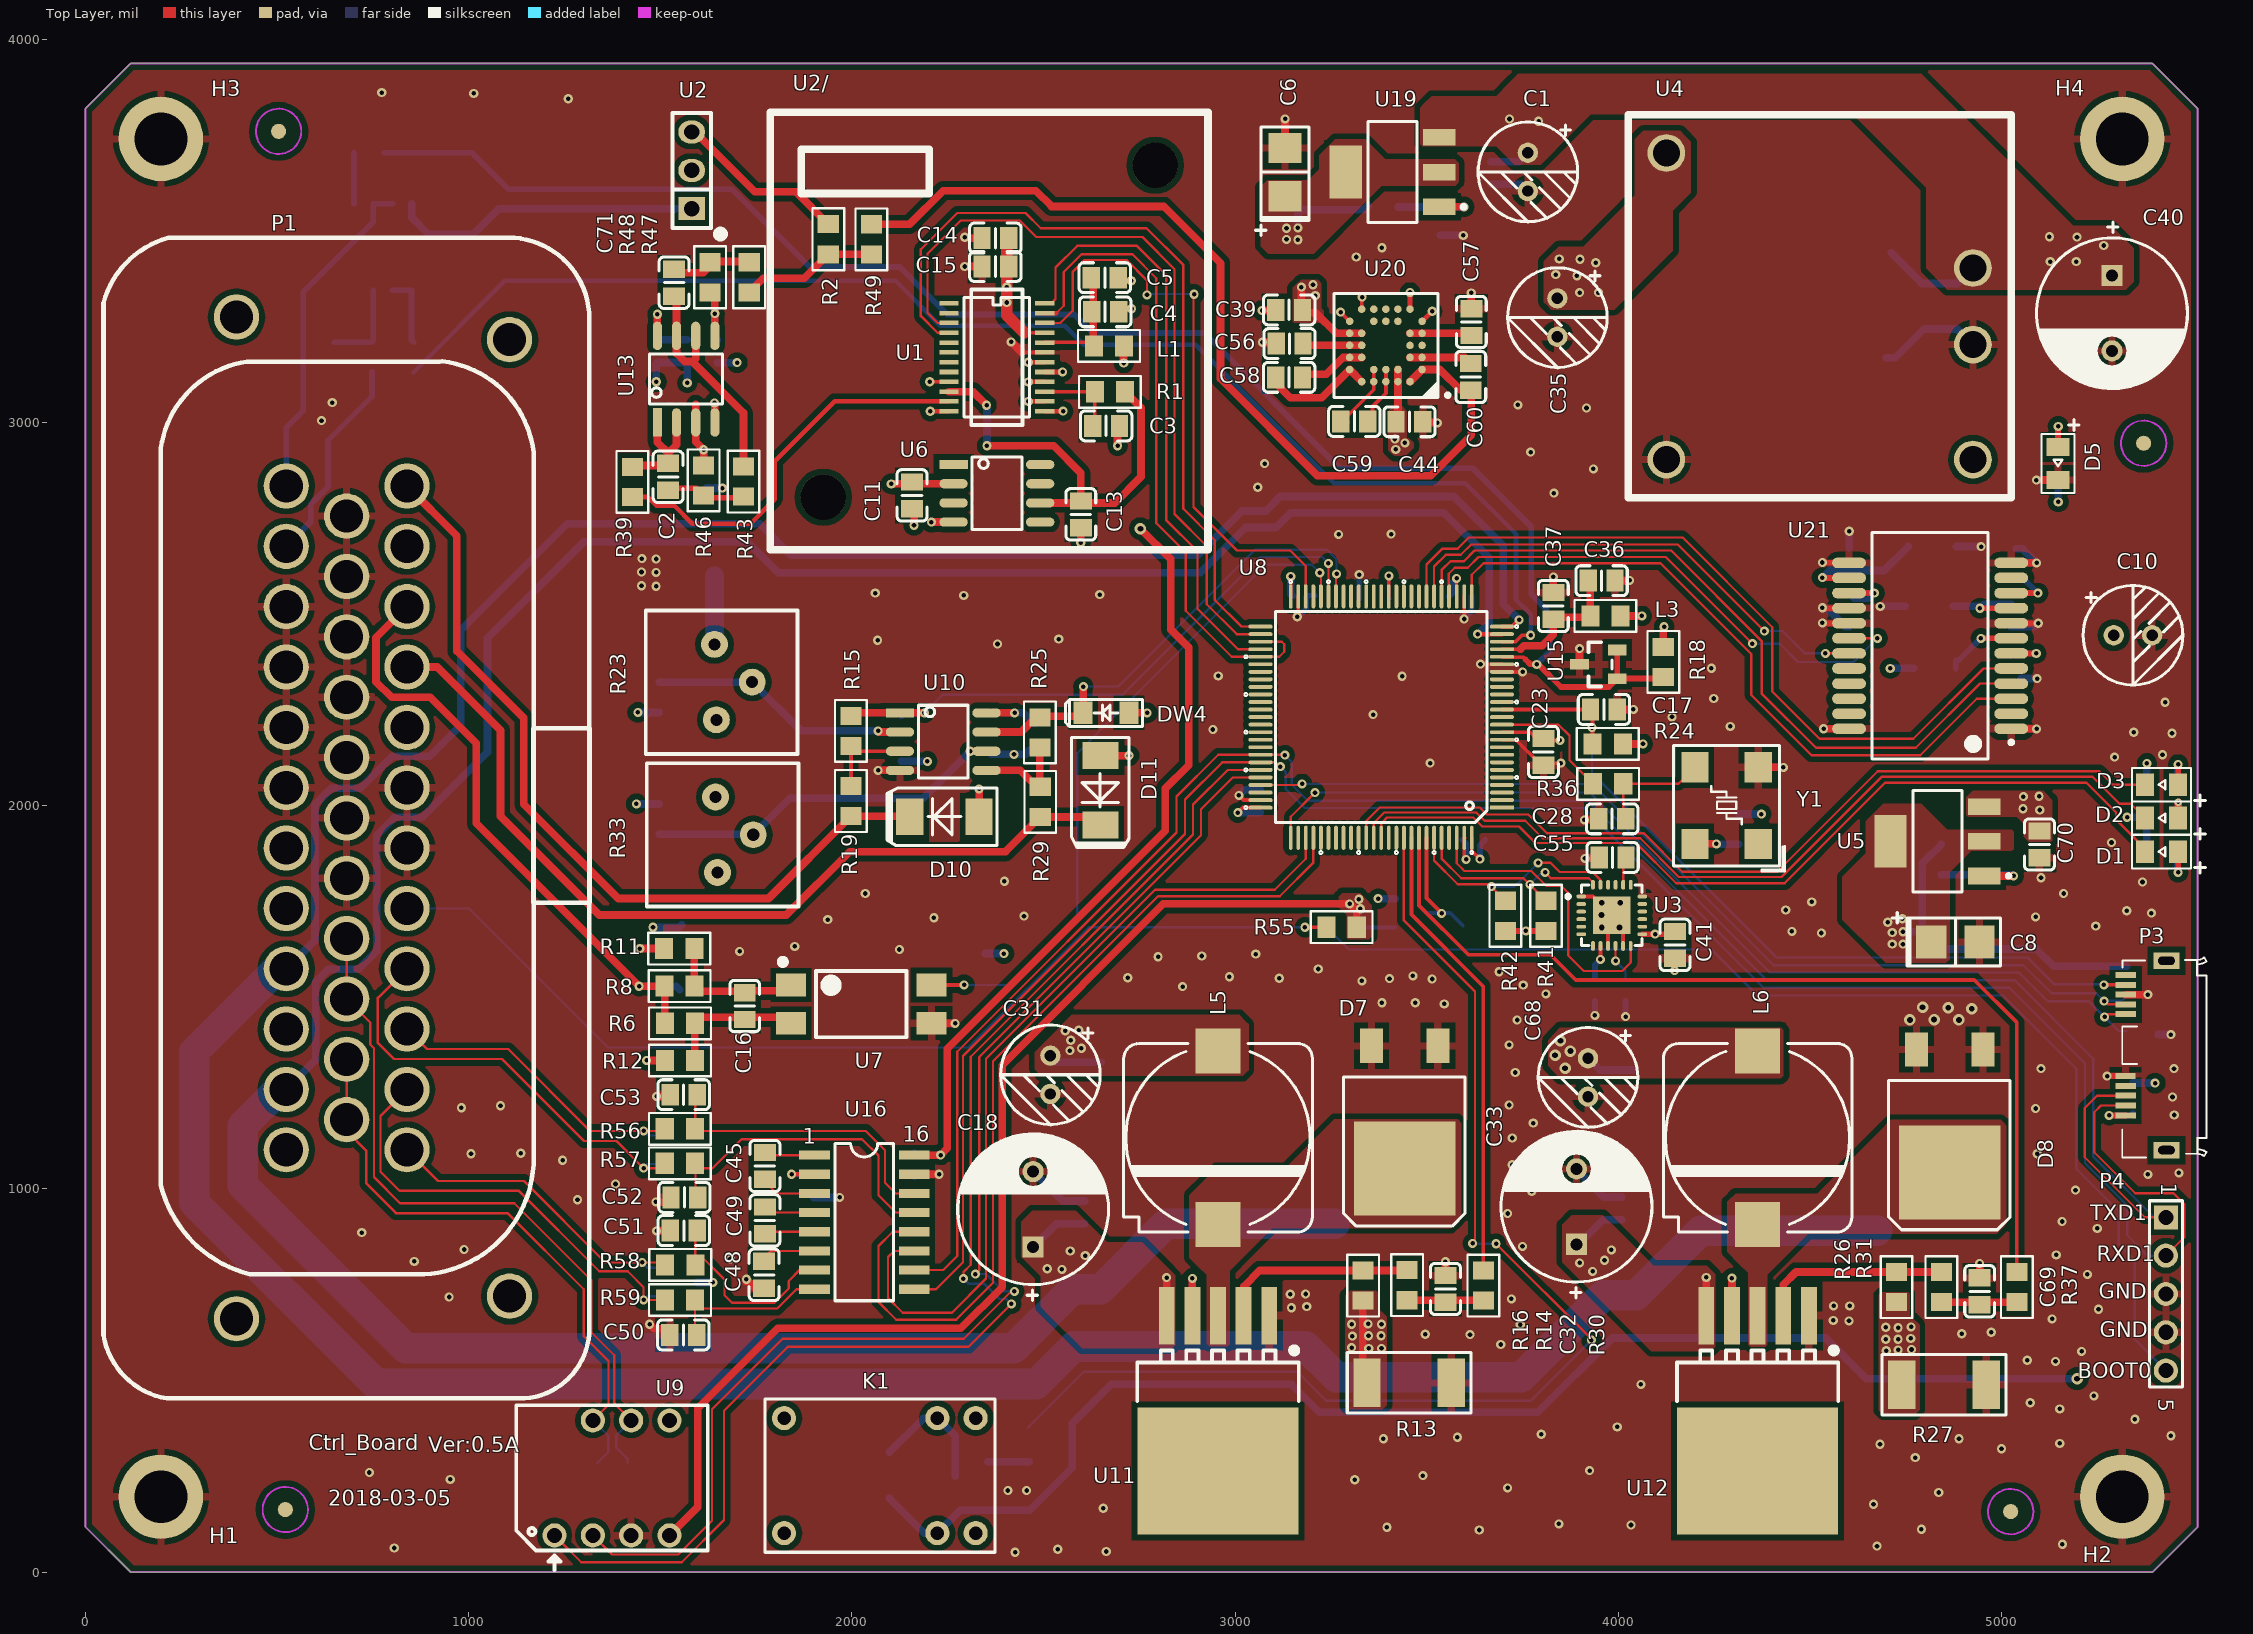
[diagram p0: Top Layer view]
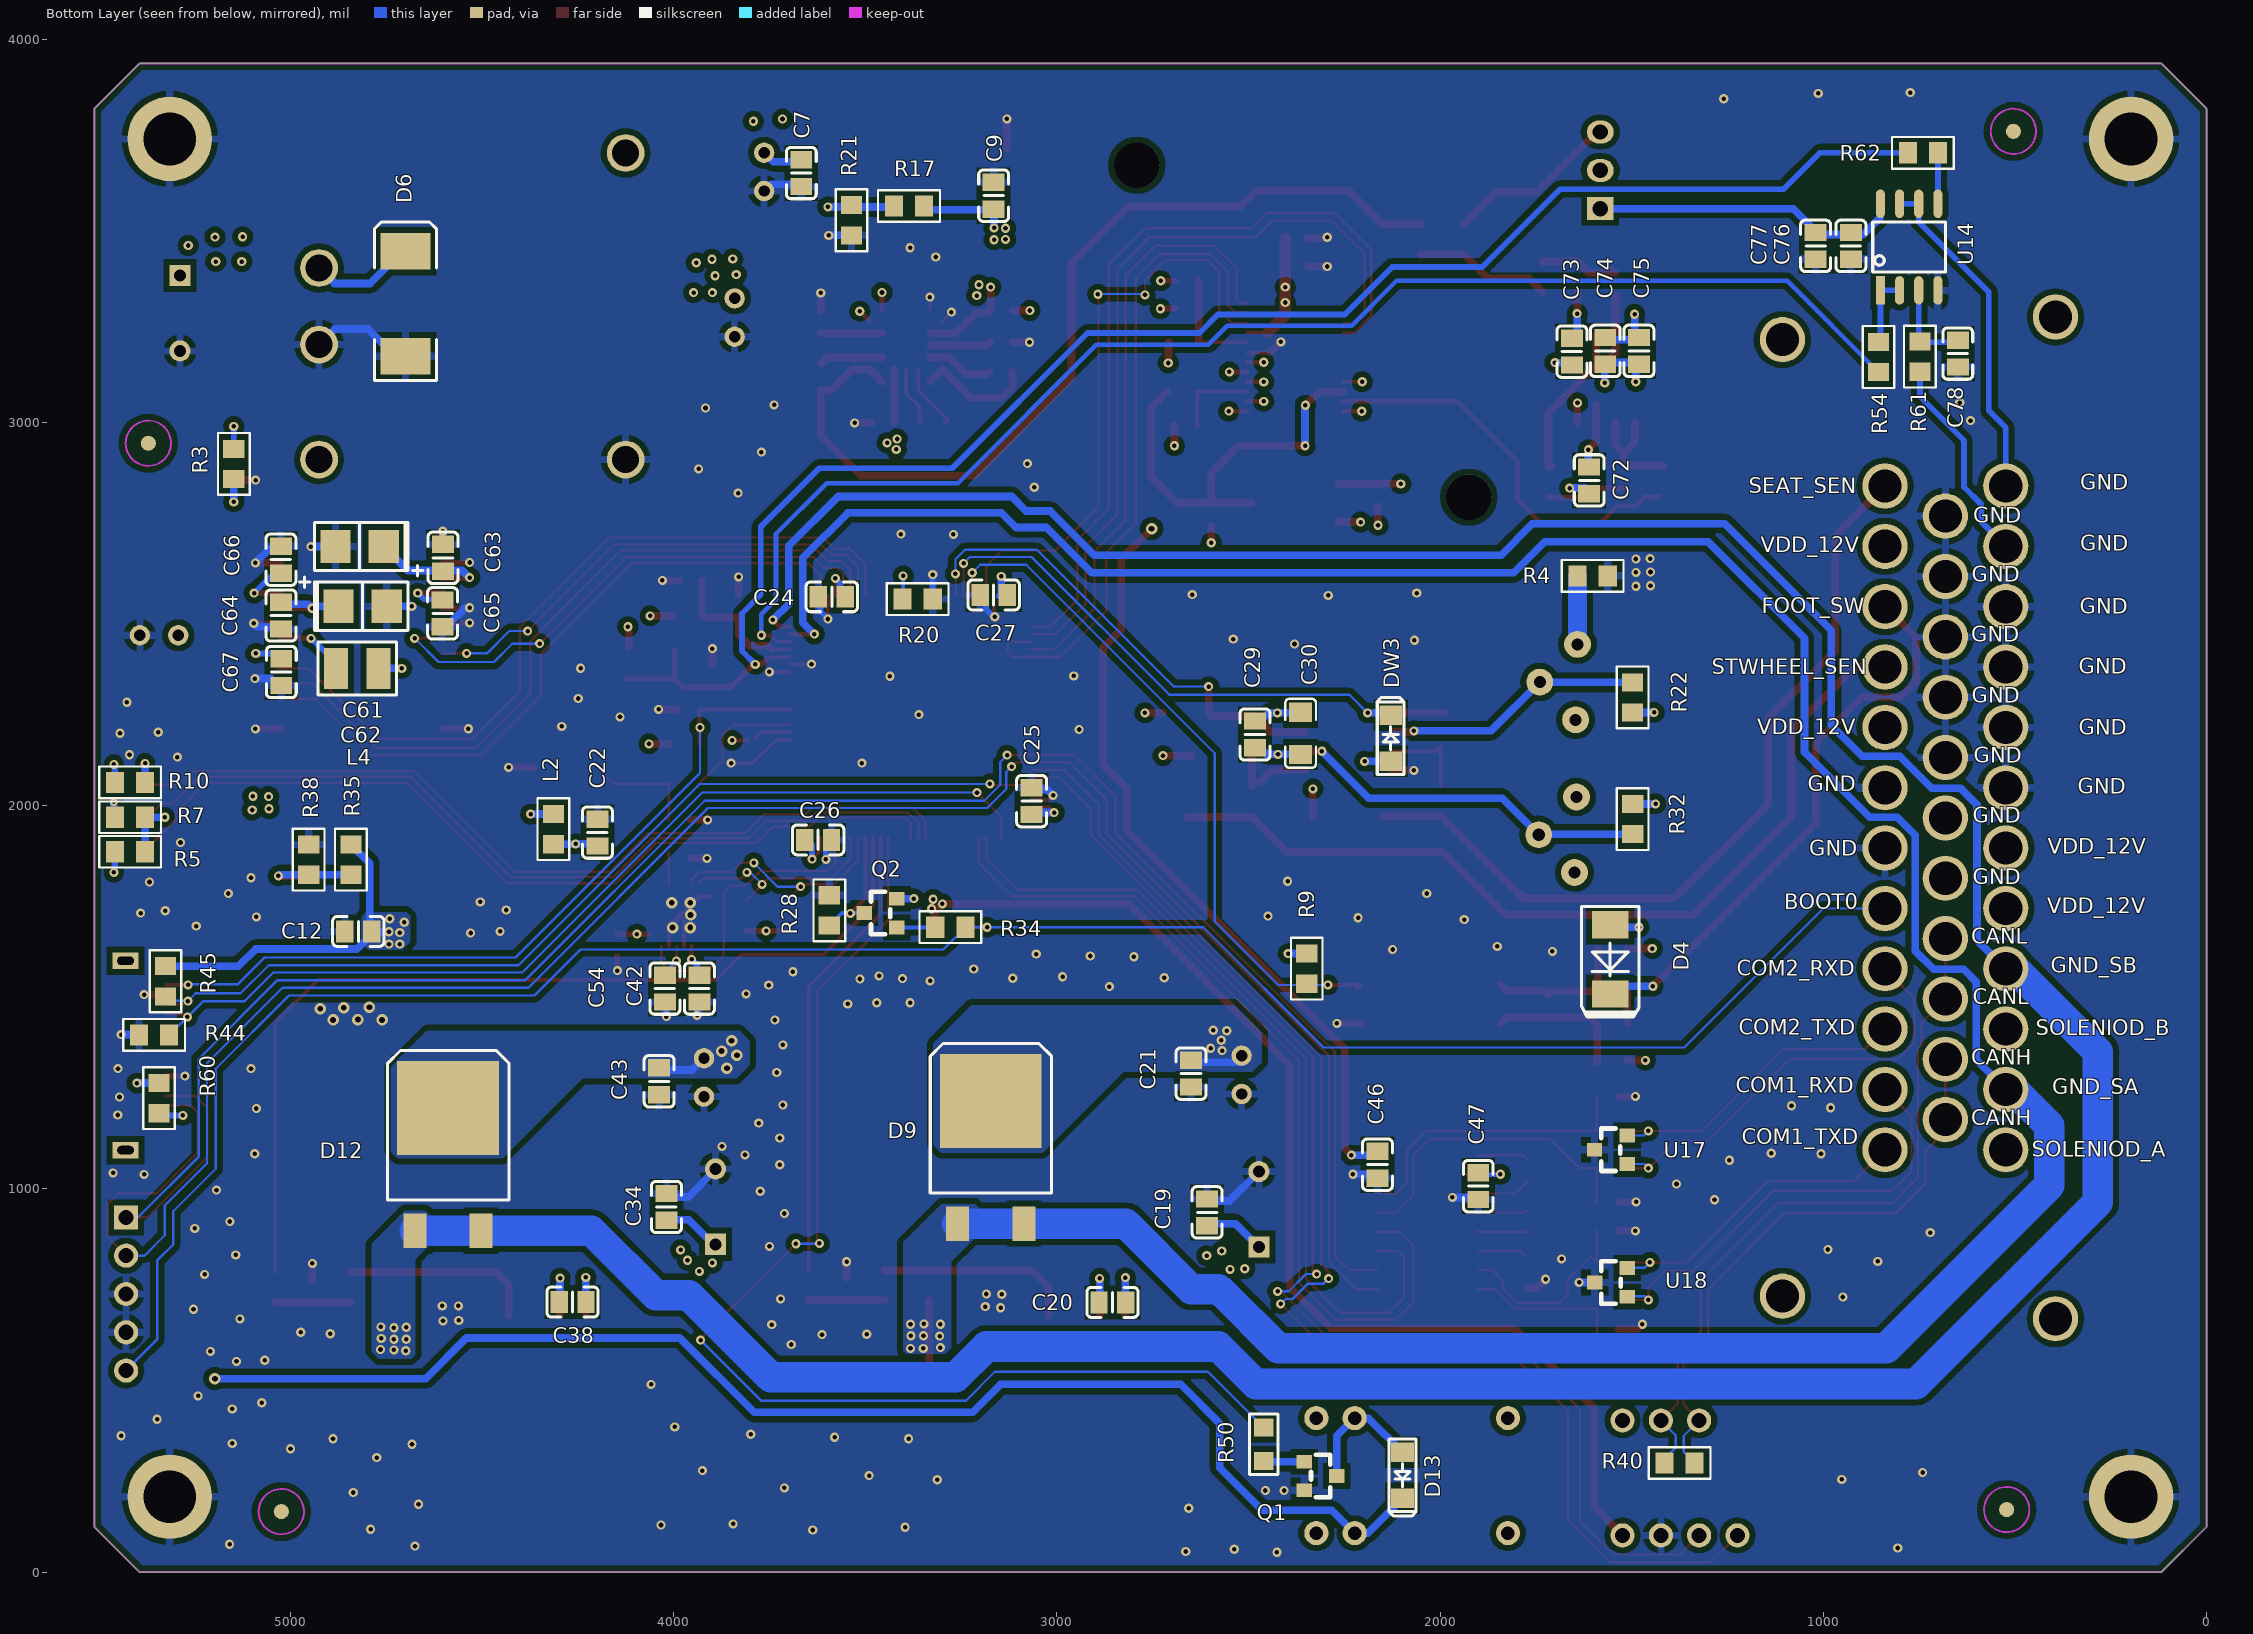
[diagram p1: Bottom Layer view, seen from below]
# Altium PCB MISC82155.PcbDoc (part 1 of 5)
Units mil, origin at the board's own origin, x right, y up, seen from the top; angles counter-clockwise.
Board outline 5511.81 x 3937.01 mil, 4 copper layers (Top Layer, GND, POWER, Bottom Layer); 191 components, 134 nets, 709 pads, 440 vias.

## Layer stack, top to bottom (the 12.6 mil dielectric is the usual default, probably not edited)
Top Layer: signal copper 1.4
Dielectric: core 12.6, FR-4, Dk 4.8
GND: plane copper 1.4, net (Multiple Nets)
Dielectric: prepreg 12.6, FR-4, Dk 4.8
POWER: plane copper 1.4, net (Multiple Nets)
Dielectric: core 12.6, FR-4, Dk 4.8
Bottom Layer: signal copper 1.4

## Board outline
0,118.11 118.11,0 5393.7,0 5511.81,118.11 5511.81,3818.9 5393.7,3937.01 118.11,3937.01 0,3818.9

## Design rules (kind name [scope] priority, off if disabled: settings)
Clearance Clearance_1 [InPolygon] p1: gap=15
Clearance [All] p2: gap=6
ComponentClearance [All] p1 off: gap=10 collisioncheckmode=3 verticalgap=10 showdistances=FALSE
HoleSize [All] p1: absolutevalues=TRUE maxlimit=196.85 minlimit=1 maxpercent=80.000 minpercent=20.000
MinimumSolderMaskSliver [All] p1 off: minsoldermaskwidth=10
PlaneClearance [All] p1: clearance=20
PlaneConnect [All] p1: planeconnectstyle=Direct reliefexpansion=20 reliefentries=4 reliefconductorwidth=10 reliefairgap=10
PolygonConnect PolygonConnect_3 [Isvia] p1: connectstyle=Direct reliefconductorwidth=10 reliefentries=4 polygonreliefangle="90 Angle"
PolygonConnect PolygonConnect_2 [InNet('AGND')] p2: connectstyle=Direct reliefconductorwidth=19.68 reliefentries=4 polygonreliefangle="90 Angle"
PolygonConnect PolygonConnect_1 [InNet('GND')] p3: connectstyle=Relief reliefconductorwidth=20 reliefentries=4 polygonreliefangle="90 Angle"
PolygonConnect [All] p4: connectstyle=Direct reliefconductorwidth=7.87 reliefentries=4 polygonreliefangle="90 Angle"
RoutingVias [All] p1: holewidth=11.81 width=23.62 viastyle="Through Hole" minholewidth=11.81 minwidth=23.62 maxholewidth=28 maxwidth=50
SilkToSilkClearance [All] p1 off: silktosilkclearance=10
SilkscreenOverComponentPads [IsPad] p1 off: minsilkscreentomaskgap=10
SolderMaskExpansion [All] p1: expansion=4
Width [All] p1: maxlimit=80 minlimit=6 preferedwidth=6 minimp=50.000000 maximp=50.000000 favimp=50.000000
21 further rules are at their usual default settings.

## Components (designator, comment, footprint, x,y, rotation, side; value= is the part's Value field where it differs from the comment)
C1 "100uF/25V" RB6.3*7 3764,3654 r270 top
C2 "22nF" C0805 1520.41,2858.34 r270 top
C3 "10nF" C0805 2663.41,2991.34 r0 top
C4 "10uF" C0805 2661,3289 r0 top
C5 "100nF" C0805 2660,3378 r0 top
C6 "47uF/10V" CT3528-B 3130.41,3653.34 r90 top
C7 "100nF" C0805 3667,3651 r90 bottom
C8 "47uF/10V" CT3528-B 4879.41,1644.34 r0 top
C9 "100nF" C0805 3165,3592 r270 bottom
C10 "100uF/25V" RB6.3*7 5343,2445 r0 top
C11 "100nF" C0805 2157,2810 r90 top
C12 "100nF" C0805 4823,1672 r180 bottom
C13 "100nF" C0805 2597.41,2760.34 r270 top
C14 "10uF" C0805 2374.41,3481.34 r180 top
C15 "100nF" C0805 2374.41,3407.34 r180 top
C16 "1μF,±10%" C0805 1720.41,1477.34 r270 top
C17 "100nF" C0805 3962.41,2251.34 r180 top
C18 "470μF/25V" CAPPR5.0-10X16-0.8 2473,947 r90 top
C19 "1uF" C0805 2608,939 r90 bottom
C20 "1uF" C0805 2855,704 r0 bottom
C21 "1uF" C0805 2650,1301 r270 bottom
C22 "100nF" C0805 4199,1930 r90 bottom
C23 "100nF" C0805 3804.41,2140.34 r270 top
C24 "100nF" C0805 3587.41,2545.34 r0 bottom
C25 "100nF" C0805 3066,2012 r90 bottom
C26 "100nF" C0805 3623,1911 r180 bottom
C27 "100nF" C0805 3165,2550 r0 bottom
C28 "15pF" C0805 3984,1966 r0 top
C29 "100nF" C0805 2483,2186 r270 bottom
C30 "4.7uF/25V" 1206C 2364,2189 r270 bottom
C31 "100uF/25V" RB6.3*7 2518,1298 r270 top
C32 "1uF" C0805 3549,739 r90 top
C33 "470μF/25V" CAPPR5.0-10X16-0.8 3891,954 r90 top
C34 "1uF" C0805 4019,953 r90 bottom
C35 "100uF/25V" RB6.3*7 3841,3274 r270 top
C36 "1μF,±10%" C0805 3956.41,2587.34 r180 top
C37 "10nF" C0805 3830.41,2521.34 r270 top
C38 "1uF" C0805 4264,705 r0 bottom
C39 "100nF" C0805 3141,3294 r0 top
C40 "330μF/35V" CAPPR5.0-10X16-0.8 5288.41,3285.34 r270 top
C41 "100nF" C0805 4148,1637 r90 top
C42 "10nF" C0805 3933,1523 r90 bottom
C43 "1uF" C0805 4038,1281 r270 bottom
C44 "100nF" C0805 3455,3002 r180 top
C45 "100nF" C0805 1773,1060 r90 top
C46 "100nF" C0805 2163.41,1063.34 r270 bottom
C47 "100nF" C0805 1900.41,1007.34 r270 bottom
C48 "100nF" C0805 1771,776 r270 top
C49 "100nF" C0805 1773,918 r90 top
C50 "15pF" C0805 1560,619 r180 top
C51 "15pF" C0805 1561.41,891.34 r180 top
C52 "15pF" C0805 1563,978 r180 top
C53 "15pF" C0805 1561,1246 r180 top
C54 "100nF" C0805 4023,1523 r90 bottom
C55 "2.2nF" C0805 3985,1865 r0 top
C56 "100nF" C0805 3142,3206 r0 top
C57 "100nF" C0805 3616.41,3262.34 r90 top
C58 "22nF" C0805 3141,3118 r0 top
C59 "22nF" C0805 3311,3003 r0 top
C60 "10nF" C0805 3615,3119 r90 top
C61 "47uF/10V" CT3528-B 4819.66,2676.41 r0 bottom
C62 "47uF/10V" CT3528-B 4811.66,2520.41 r180 bottom
C63 "1uF" C0805 4602,2647 r90 bottom
C64 "100nF" C0805 5024.66,2496.41 r270 bottom
C65 "1uF" C0805 4603,2502 r270 bottom
C66 "1uF" C0805 5025,2642 r90 bottom
C67 "470nF" C0805 5024,2349 r270 bottom
C68 "100uF/25V" RB6.3*7 3921,1291 r270 top
C69 "1uF" C0805 4943,733 r90 top
C70 "100nF" C0805 5099,1899 r90 top
C71 "22nF" C0805 1536,3365 r90 top
C72 "22nF" C0805 1611,2849 r270 bottom
C73 "22nF" C0805 1656,3185 r270 bottom
C74 "10uF" C0805 1569,3187 r270 bottom
C75 "100nF" C0805 1481,3187 r270 bottom
C76 "10uF" C0805 928,3461 r270 bottom
C77 "100nF" C0805 1020,3461 r270 bottom
C78 "100nF" C0805 649,3180 r270 bottom
D1 "LED0-RED" LED0805 5417.69,1880 r180 top
D2 "LED0-GREEN" LED0805 5417.69,1968 r180 top
D3 "LED0-BLUE" LED0805 5417.69,2055 r180 top
D4 "P6SMB15A" DO-214 1556,1599 r270 bottom
D5 "LED0-RED" LED0805 5147.41,2893.34 r270 top
D6 "SMCJ18A" SMC 4700,3310 r90 bottom
D7 "MBRD1045" TO-252 3442.41,1373.34 r180 top
D8 "MBRD1045" TO-252 4865,1364 r180 top
D9 "MBRD1045" TO-252 3173,909 r180 bottom
D10 "P6SMB15A" DO-214 2241.41,1971.34 r180 top
D11 "P6SMB15A" DO-214 2648.41,2040.34 r270 top
D12 "MBRD1045" TO-252 4589,891 r180 bottom
D13 "1N4148" SMD-D4148 2098,253 r270 bottom
DW3 "ZMM3V3" SMD-D4148 2129,2176 r90 bottom
DW4 "ZMM3V3" SMD-D4148 2663.41,2242.34 r180 top
H1 "Hole" HOLE-3.2 196.85,196.85 r0 top
H2 "Hole" HOLE-3.2 5314.96,196.85 r0 top
H3 "Hole" HOLE-3.2 196.85,3740.16 r0 top
H4 "Hole" HOLE-3.2 5314.96,3740.16 r0 top
K1 "HK4100F-DC5V-SHG 0.2W" HK4100F 2323,402 r180 top
L1 "1uH" R0805 2671,3200 r180 top
L2 "1uH" R0805 4314,1939 r90 bottom
L3 "10uH" R0805 3966.41,2495.34 r180 top
L4 "47uH" R1210 4825.66,2358.41 r0 bottom
L5 "33uH" SLF12555 2955.41,1133.34 r90 top
L6 "33uH" SLF12555 4363.41,1133.34 r90 top
P1 "CON 35-776230-1" VGA35 750.41,1968.34 r270 top locked
P3 "USB3.0-B" "Micro USB3.0-B" 5430.46,1101.34 r90 top
P4 "2.54 single-row pin header" HDR1X5 5429,726 r270 top
Q1 "SS8050LT(1.5A)" SOT-23 2312,251 r180 bottom
Q2 "8550" SOT-23 3460.15,1720 r0 bottom
R1 "0R" R0805 2673.41,3080.34 r0 top
R2 "0R" R0805 1938.41,3478.34 r90 top
R3 "2K" R0805 5148,2892 r270 bottom
R4 "0R" R0805 1602,2600 r180 bottom
R5 "1K" R0805 5418.69,1880 r180 bottom
R6 "2K" R0805 1551.41,1432.34 r0 top
R7 "1K" R0805 5418.69,1970 r180 bottom
R8 "2K" R0805 1550.41,1529.34 r0 top
R9 "10K" R0805 2348,1575 r270 bottom
R10 "1K" R0805 5418.69,2061 r180 bottom
R11 "10K" R0805 1549.41,1627.34 r180 top
R12 "10K" R0805 1551.41,1335.34 r180 top
R13 "0.08R" R2512 3454,494 r180 top
R14 "14K" R0805 3449,749 r270 top
R15 "100K" R0805 1997.41,2195.34 r270 top
R16 "1K" R0805 3334,748 r90 top
R17 "10K" R0805 3386,3565 r180 bottom
R18 "1K" R0805 4117.41,2375.34 r270 top
R19 "10K" R0805 1997.41,2012.34 r270 top
R20 "10K" R0805 3363.41,2539.34 r0 bottom
R21 "38.3K" R0805 3536,3528 r90 bottom
R22 "100K" R0805 1497.62,2282.77 r270 bottom
R23 "100KΩ potentiometer" CHANGER3 1690.62,2322.77 r270 top
R24 "10K" R0805 3972.41,2161.34 r0 top
R25 "100K" R0805 2490.41,2191.34 r270 top
R26 "1K" R0805 4726,744 r90 top
R27 "0.08R" R2512 4850,489 r180 top
R28 "10K" R0805 3594,1727 r270 bottom
R29 "10K" R0805 2491.53,2010.23 r270 top
R30 "1K" R0805 3648,748 r270 top
R31 "14K" R0805 4843,744 r270 top
R32 "100K" R0805 1497.41,1965.34 r90 bottom
R33 "100KΩ potentiometer" CHANGER3 1693.41,1924.34 r270 top
R34 "10K" R0805 3278,1683 r180 bottom
R35 "1K" R0805 4842.41,1859.34 r90 bottom
R36 "10R" R0805 3973.41,2057.34 r0 top
R37 "1K" R0805 5040,744 r270 top
R38 "1.6K" R0805 4952.41,1859.34 r270 bottom
R39 "0R" R0805 1427,2845 r270 top
R40 "120R" R0805 1375,285 r0 bottom
R41 "10K" R0805 3811.32,1712.81 r270 top
R42 "10K" R0805 3705.32,1712.81 r270 top
R43 "56K 1%" R0805 1717,2846 r270 top
R44 "10K" R0805 5356,1402 r180 bottom
R45 "10K" R0805 5326,1542 r270 bottom
R46 "91K 1%" R0805 1613,2849 r90 top
R47 "56K 1%" R0805 1732,3379 r90 top
R48 "91K 1%" R0805 1630,3379 r270 top
R49 "0R" R0805 2051,3478 r90 top
R50 "1kΩ,±1%" 0805R 2460,334 r270 bottom
R54 "0R" R0805 856,3171 r270 bottom
R55 "10K" R0805 3278,1683 r0 top
R56 "4.7R" R0805 1551,1157 r180 top
R57 "4.7R" R0805 1551,1067 r180 top
R58 "4.7R" R0805 1552,802 r180 top
R59 "4.7R" R0805 1551.41,710.34 r180 top
R60 "0R" R0805 5343,1237 r270 bottom
R61 "10K" R0805 748,3172 r270 bottom
R62 "0R" R0805 740,3704 r180 bottom
U1 "AD7190BRUZ" IC-24P-TSSOP-6_4MM-G 2378.41,3170.34 r270 top
U2 "CRS03" HDR1X3 1582,3658 r90 top
U2/ "CRS03" CDS43-01 2358.41,3238.34 r90 top locked
U3 "MPU6050" QFN24 3983,1714 r0 top
U4 "E2405UHBDD-10W" E2403UHBDD 4525.41,3303.34 r180 top
U5 "1117-ADJ" SOT-223 4832.41,1907.34 r90 top
U6 "ADR03A" SOP-8 2378.41,2815.34 r270 top
U7 "PC817" SMD-4 2024.41,1482.34 r0 top
U8 "STM32F103VCT6" QFP-100 3381.41,2231.34 r180 top
U9 "CTM1051AM" CTM1051AM 1374,246 r0 top
U10 "LM293DR" SOP-8 2238.41,2167.34 r270 top
U11 "XL3005" TO-263-5 2955.41,669.34 r90 top
U12 "XL3005" TO-263-5 4363.41,669.34 r90 top
U13 "AD8616ARZ" SOP-8 1567.41,3113.34 r0 top
U14 "LMV358IDR" SOP-8 776,3458 r180 bottom
U15 "TL431AQDBZT" LC-SOT-23(SOT-23-3) 3948,2369 r0 top
U16 "SP3232EEN" SOP16-6.6 2032.41,913.34 r0 top
U17 "PESD15VL2BT" SOT-23 1554.41,1102.34 r0 bottom
U18 "PESD15VL2BT" SOT-23 1554,756 r0 bottom
U19 "1117-ADJ" SOT-223 3410.28,3653.46 r90 top
U20 "ADXRS646" ADXRS646 3393.41,3201.34 r180 top
U21 "SCC2130" SCC2130D 4813.78,2417.29 r180 top
Y1 "8MHZ 3.3V 20PPM" XTAL7050 4282.41,2000.34 r90 top

## Footprints (in the part's own frame and the unit in brackets; to place one, negate y for a bottom-side part, rotate by r counter-clockwise, add the part's x,y. Pads: shape width x height; smd on the part's side, far side on the other; paste and mask are expansions set on the pad)
0805R [mm]
  rect 1.2x1.3 smd: 1(-1.118,0) 2(1.118,0)
  silkscreen extent -2,-0.95 2,0.95
1206C [mil]
  rect 50x60 smd: 1(-55,0) 2(55,0)
  silkscreen extent -90,-40 90,40, body extent -62,-32 64,31, height 39
ADXRS646 [mm] "BGA, 32-Leads, Body 6.88x6.88mmx3.80mm, Pitch 0.80mm"
  round 0.5 smd: A2(-1.6,2.4) A3(-0.8,2.4) A4(0,2.4) A5(0.8,2.4) A6(1.6,2.4) B1(-2.4,1.6) B3(-0.8,1.6) B4(0,1.6) B5(0.8,1.6) B7(2.4,1.6) C1(-2.4,0.8) C2(-1.6,0.8) C6(1.6,0.8) C7(2.4,0.8) D1(-2.4,0) D2(-1.6,0) D6(1.6,0) D7(2.4,0) E1(-2.4,-0.8) E2(-1.6,-0.8) E6(1.6,-0.8) E7(2.4,-0.8) F1(-2.4,-1.6) F3(-0.8,-1.6) F4(0,-1.6) F5(0.8,-1.6) F7(2.4,-1.6) G2(-1.6,-2.4) G3(-0.8,-2.4) G4(0,-2.4) G5(0.8,-2.4) G6(1.6,-2.4)
  silkscreen extent -4.23,-3.45 3.45,3.45, body extent -3.44,-3.44 3.44,3.44, height 3.8
C0805 [mm] "Chip Capacitor, Body 2.0x1.3mm, IPC High Density"
  rect 1.15x1.45 smd: 1(-0.889,0) 2(0.889,0)
  silkscreen extent -1.7,-0.99 1.7,0.99, body extent -1,-0.63 1,0.63, height 0.78
CAPPR5.0-10X16-0.8 [mm]
  rect 1.4x1.4 hole 0.8: 1(-2.5,0)
  round 1.4 hole 0.8: 2(2.5,0)
  silkscreen extent -6.05,-5 5,5, body extent -5.1,-5.1 4.9,4.9, height 15.68
CDS43-01 [mm]
  round 3 hole 3: 1(-11,11) 2(11,-11)
  silkscreen extent -14.5,-14.5 14.5,14.5
CHANGER3 [mm]
  round 1.778 hole 0.8: 1(-2.5,-1.25) 2(0,1.25) 3(2.5,-1.123)
  silkscreen extent -4.73,-5.81 4.77,4.25
CT3528-B [mm]
  rect 2x2.2 smd: 1(-1.6,0) 2(1.6,0)
  silkscreen extent -4.2,-1.6 3,1.95, body extent -1.75,-1.4 1.75,1.4, height 1.9